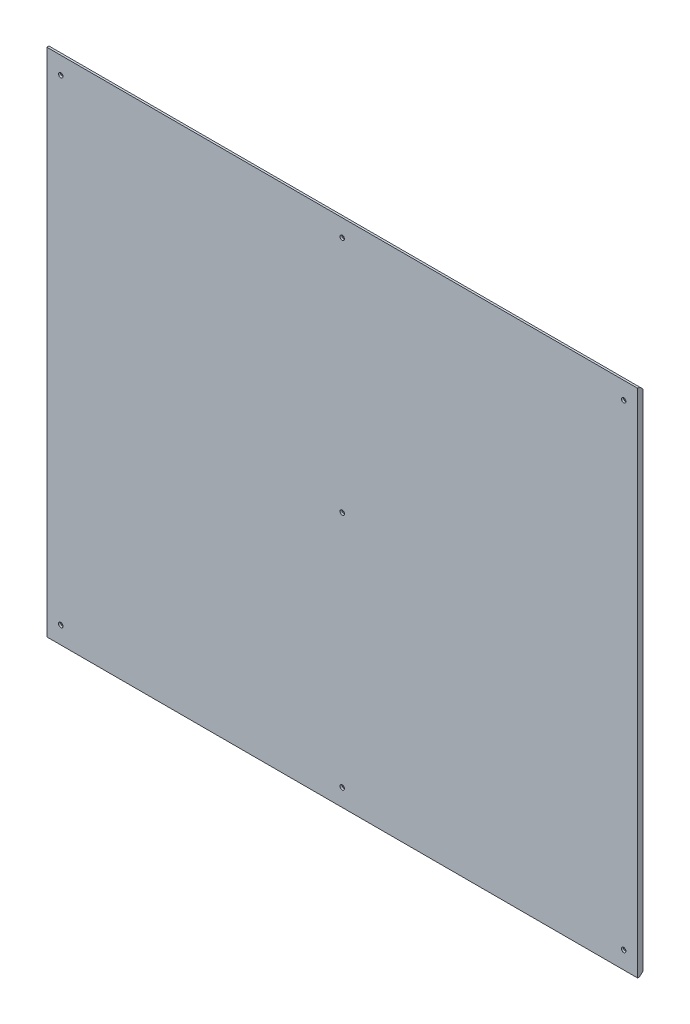
from build123d import *

# Parameters (mm, degrees)
SKETCH_1_W                    = 850
SKETCH_1_H                    = 735
EXTRUDE_1_DEPTH               = 8
CHAMFER_1_SIZE                = 5
SKETCH_2_R                    = 8.25
CUT_EXTRUDE_1_DEPTH           = 5
CUT_EXTRUDE_1_DRAFT           = -45
CUT_EXTRUDE_1_PROFILE_2_DEPTH = 5
CUT_EXTRUDE_1_PROFILE_2_DRAFT = -45
CUT_EXTRUDE_1_PROFILE_3_DEPTH = 5
CUT_EXTRUDE_1_PROFILE_3_DRAFT = -45
CUT_EXTRUDE_1_PROFILE_4_DEPTH = 5
CUT_EXTRUDE_1_PROFILE_4_DRAFT = -45
CUT_EXTRUDE_1_PROFILE_5_DEPTH = 5
CUT_EXTRUDE_1_PROFILE_5_DRAFT = -45
CUT_EXTRUDE_1_PROFILE_6_DEPTH = 5
CUT_EXTRUDE_1_PROFILE_6_DRAFT = -45
SKETCH_3_R                    = 3.25
CUT_EXTRUDE_2_DEPTH           = 3
SKETCH_4_R                    = 8.25
CUT_EXTRUDE_3_DEPTH           = 5
CUT_EXTRUDE_3_DRAFT           = -45
SKETCH_5_R                    = 3.25
CUT_EXTRUDE_4_DEPTH           = 5


with BuildPart() as part:
    # 草图1 → 凸台-拉伸1 (new body)
    with BuildSketch(Plane.XY):
        Rectangle(SKETCH_1_W, SKETCH_1_H)
    extrude(amount=EXTRUDE_1_DEPTH)

    # 倒角1
    chamfer_1_edges = [part.edges().sort_by_distance(p)[0] for p in [
        (0, -367.5, 0),
        (0, 367.5, 0),
    ]]
    chamfer(chamfer_1_edges, length=CHAMFER_1_SIZE)


with BuildPart() as cut_extrude_1_tool:
    # 草图2 → 切除-拉伸1 (with draft: the straight prism first)
    with BuildSketch(Plane(origin=(0, 0, 0), x_dir=(-1, 0, 0), z_dir=(0, 0, -1))):
        with Locations((-405, 342.5)):
            Circle(SKETCH_2_R)
    extrude(amount=-CUT_EXTRUDE_1_DEPTH)
    # 切除-拉伸1: the draft: its side faces are tilted about the plane it starts from
    cut_extrude_1_sides = [cut_extrude_1_tool.faces().sort_by_distance(p)[0] for p in [
        (413.25, 342.5, 2.5),
    ]]
    draft(cut_extrude_1_sides, Plane(origin=(0, 0, 0), x_dir=(-1, 0, 0), z_dir=(0, 0, -1)), CUT_EXTRUDE_1_DRAFT)


with BuildPart() as part_1:
    add(part.part)

    # 切除-拉伸1: cut by cut_extrude_1_tool
    add(cut_extrude_1_tool.part, mode=Mode.SUBTRACT)


with BuildPart() as cut_extrude_1_profile_2_tool:
    # 草图2 → 切除-拉伸1 profile 2 (with draft: the straight prism first)
    with BuildSketch(Plane(origin=(0, 0, 0), x_dir=(-1, 0, 0), z_dir=(0, 0, -1))):
        with Locations((0, 342.5)):
            Circle(SKETCH_2_R)
    extrude(amount=-CUT_EXTRUDE_1_PROFILE_2_DEPTH)
    # 切除-拉伸1 profile 2: the draft: its side faces are tilted about the plane it starts from
    cut_extrude_1_profile_2_sides = [cut_extrude_1_profile_2_tool.faces().sort_by_distance(p)[0] for p in [
        (8.25, 342.5, 2.5),
    ]]
    draft(cut_extrude_1_profile_2_sides, Plane(origin=(0, 0, 0), x_dir=(-1, 0, 0), z_dir=(0, 0, -1)), CUT_EXTRUDE_1_PROFILE_2_DRAFT)


with BuildPart() as part_2:
    add(part_1.part)

    # 切除-拉伸1 profile 2: cut by cut_extrude_1_profile_2_tool
    add(cut_extrude_1_profile_2_tool.part, mode=Mode.SUBTRACT)


with BuildPart() as cut_extrude_1_profile_3_tool:
    # 草图2 → 切除-拉伸1 profile 3 (with draft: the straight prism first)
    with BuildSketch(Plane(origin=(0, 0, 0), x_dir=(-1, 0, 0), z_dir=(0, 0, -1))):
        with Locations((405, 342.5)):
            Circle(SKETCH_2_R)
    extrude(amount=-CUT_EXTRUDE_1_PROFILE_3_DEPTH)
    # 切除-拉伸1 profile 3: the draft: its side faces are tilted about the plane it starts from
    cut_extrude_1_profile_3_sides = [cut_extrude_1_profile_3_tool.faces().sort_by_distance(p)[0] for p in [
        (-396.75, 342.5, 2.5),
    ]]
    draft(cut_extrude_1_profile_3_sides, Plane(origin=(0, 0, 0), x_dir=(-1, 0, 0), z_dir=(0, 0, -1)), CUT_EXTRUDE_1_PROFILE_3_DRAFT)


with BuildPart() as part_3:
    add(part_2.part)

    # 切除-拉伸1 profile 3: cut by cut_extrude_1_profile_3_tool
    add(cut_extrude_1_profile_3_tool.part, mode=Mode.SUBTRACT)


with BuildPart() as cut_extrude_1_profile_4_tool:
    # 草图2 → 切除-拉伸1 profile 4 (with draft: the straight prism first)
    with BuildSketch(Plane(origin=(0, 0, 0), x_dir=(-1, 0, 0), z_dir=(0, 0, -1))):
        with Locations((-405, -342.5)):
            Circle(SKETCH_2_R)
    extrude(amount=-CUT_EXTRUDE_1_PROFILE_4_DEPTH)
    # 切除-拉伸1 profile 4: the draft: its side faces are tilted about the plane it starts from
    cut_extrude_1_profile_4_sides = [cut_extrude_1_profile_4_tool.faces().sort_by_distance(p)[0] for p in [
        (413.25, -342.5, 2.5),
    ]]
    draft(cut_extrude_1_profile_4_sides, Plane(origin=(0, 0, 0), x_dir=(-1, 0, 0), z_dir=(0, 0, -1)), CUT_EXTRUDE_1_PROFILE_4_DRAFT)


with BuildPart() as part_4:
    add(part_3.part)

    # 切除-拉伸1 profile 4: cut by cut_extrude_1_profile_4_tool
    add(cut_extrude_1_profile_4_tool.part, mode=Mode.SUBTRACT)


with BuildPart() as cut_extrude_1_profile_5_tool:
    # 草图2 → 切除-拉伸1 profile 5 (with draft: the straight prism first)
    with BuildSketch(Plane(origin=(0, 0, 0), x_dir=(-1, 0, 0), z_dir=(0, 0, -1))):
        with Locations((0, -342.5)):
            Circle(SKETCH_2_R)
    extrude(amount=-CUT_EXTRUDE_1_PROFILE_5_DEPTH)
    # 切除-拉伸1 profile 5: the draft: its side faces are tilted about the plane it starts from
    cut_extrude_1_profile_5_sides = [cut_extrude_1_profile_5_tool.faces().sort_by_distance(p)[0] for p in [
        (8.25, -342.5, 2.5),
    ]]
    draft(cut_extrude_1_profile_5_sides, Plane(origin=(0, 0, 0), x_dir=(-1, 0, 0), z_dir=(0, 0, -1)), CUT_EXTRUDE_1_PROFILE_5_DRAFT)


with BuildPart() as part_5:
    add(part_4.part)

    # 切除-拉伸1 profile 5: cut by cut_extrude_1_profile_5_tool
    add(cut_extrude_1_profile_5_tool.part, mode=Mode.SUBTRACT)


with BuildPart() as cut_extrude_1_profile_6_tool:
    # 草图2 → 切除-拉伸1 profile 6 (with draft: the straight prism first)
    with BuildSketch(Plane(origin=(0, 0, 0), x_dir=(-1, 0, 0), z_dir=(0, 0, -1))):
        with Locations((405, -342.5)):
            Circle(SKETCH_2_R)
    extrude(amount=-CUT_EXTRUDE_1_PROFILE_6_DEPTH)
    # 切除-拉伸1 profile 6: the draft: its side faces are tilted about the plane it starts from
    cut_extrude_1_profile_6_sides = [cut_extrude_1_profile_6_tool.faces().sort_by_distance(p)[0] for p in [
        (-396.75, -342.5, 2.5),
    ]]
    draft(cut_extrude_1_profile_6_sides, Plane(origin=(0, 0, 0), x_dir=(-1, 0, 0), z_dir=(0, 0, -1)), CUT_EXTRUDE_1_PROFILE_6_DRAFT)


with BuildPart() as part_6:
    add(part_5.part)

    # 切除-拉伸1 profile 6: cut by cut_extrude_1_profile_6_tool
    add(cut_extrude_1_profile_6_tool.part, mode=Mode.SUBTRACT)

    # 草图3 → 切除-拉伸2 (cut)
    with BuildSketch(Plane.XY.offset(8)):
        with Locations((-405, 342.5)):
            Circle(SKETCH_3_R)
        with Locations((0, 342.5)):
            Circle(SKETCH_3_R)
        with Locations((405, 342.5)):
            Circle(SKETCH_3_R)
        with Locations((-405, -342.5)):
            Circle(SKETCH_3_R)
        with Locations((0, -342.5)):
            Circle(SKETCH_3_R)
        with Locations((405, -342.5)):
            Circle(SKETCH_3_R)
    extrude(amount=-CUT_EXTRUDE_2_DEPTH, mode=Mode.SUBTRACT)


with BuildPart() as cut_extrude_3_tool:
    # 草图4 → 切除-拉伸3 (with draft: the straight prism first)
    with BuildSketch(Plane(origin=(0, 0, 0), x_dir=(-1, 0, 0), z_dir=(0, 0, -1))):
        Circle(SKETCH_4_R)
    extrude(amount=-CUT_EXTRUDE_3_DEPTH)
    # 切除-拉伸3: the draft: its side faces are tilted about the plane it starts from
    cut_extrude_3_sides = [cut_extrude_3_tool.faces().sort_by_distance(p)[0] for p in [
        (8.25, 0, 2.5),
    ]]
    draft(cut_extrude_3_sides, Plane(origin=(0, 0, 0), x_dir=(-1, 0, 0), z_dir=(0, 0, -1)), CUT_EXTRUDE_3_DRAFT)


with BuildPart() as part_7:
    add(part_6.part)

    # 切除-拉伸3: cut by cut_extrude_3_tool
    add(cut_extrude_3_tool.part, mode=Mode.SUBTRACT)

    # 草图5 → 切除-拉伸4 (cut)
    with BuildSketch(Plane(origin=(0, 0, 5), x_dir=(-1, 0, 0), z_dir=(0, 0, -1))):
        Circle(SKETCH_5_R)
    extrude(amount=-CUT_EXTRUDE_4_DEPTH, mode=Mode.SUBTRACT)


solid = part_7.part
